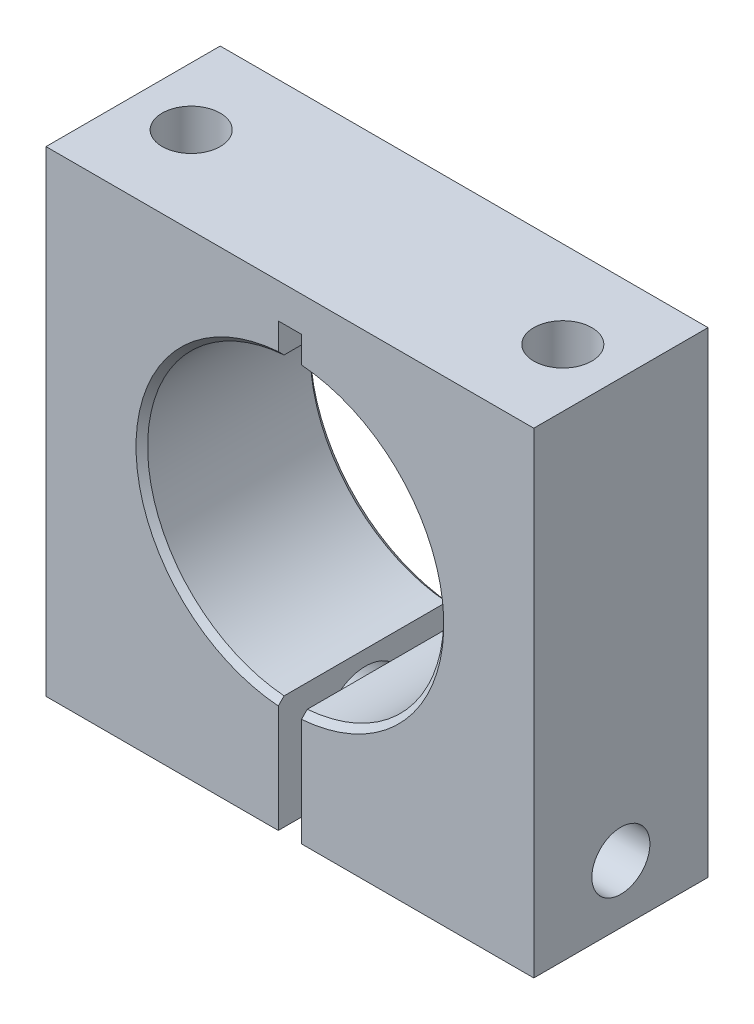
from build123d import *

# Parameters (mm, degrees)
SKETCH_1_W                = 42
SKETCH_1_H                = 41
EXTRUDE_1_DEPTH           = 15
SKETCH_2_R                = 12.75
CUT_EXTRUDE_1_DEPTH       = 15
SKETCH_3_W                = 2
SKETCH_3_H                = 38
CUT_EXTRUDE_2_DEPTH       = 15
HOLE_WIZARD_M6_1_D        = 5
HOLE_WIZARD_M6_1_DEPTH    = 17
HOLE_WIZARD_M6_1_TIP      = 1.502151548
HOLE_WIZARD_7_0_7_1_D     = 7
HOLE_WIZARD_7_0_7_1_DEPTH = 20
HOLE_WIZARD_M6_2_D        = 5
CHAMFER_1_SIZE            = 0.5
CHAMFER_2_SIZE            = 0.5


with BuildPart() as part:
    # 草图1 → 凸台-拉伸1 (new body)
    with BuildSketch(Plane.XY):
        with Locations((21, 20.5)):
            Rectangle(SKETCH_1_W, SKETCH_1_H)
    extrude(amount=EXTRUDE_1_DEPTH)

    # 草图2 → 切除-拉伸1 (cut)
    with BuildSketch(Plane.XY.offset(15)):
        with Locations((21, 22.5)):
            Circle(SKETCH_2_R)
    extrude(amount=-CUT_EXTRUDE_1_DEPTH, mode=Mode.SUBTRACT)

    # 草图3 → 切除-拉伸2 (cut)
    with BuildSketch(Plane.XY.offset(15)):
        with Locations((21, 19)):
            Rectangle(SKETCH_3_W, SKETCH_3_H)
    extrude(amount=-CUT_EXTRUDE_2_DEPTH, mode=Mode.SUBTRACT)

    # M6 螺纹孔1
    with Locations(Plane(origin=(0, 41, 0), x_dir=(1, 0, 0), z_dir=(0, 1, 0))):
        with Locations((5, -7.5), (37, -7.5)):
            Hole(HOLE_WIZARD_M6_1_D / 2, depth=HOLE_WIZARD_M6_1_DEPTH)
            with Locations((0, 0, -(HOLE_WIZARD_M6_1_DEPTH + HOLE_WIZARD_M6_1_TIP / 2))):  # 118° drill point
                Cone(0, HOLE_WIZARD_M6_1_D / 2, HOLE_WIZARD_M6_1_TIP, mode=Mode.SUBTRACT)

    # Ø7.0 (7) 直径孔1
    with Locations(Plane.ZY):
        with Locations((7.5, 5)):
            Hole(HOLE_WIZARD_7_0_7_1_D / 2, depth=HOLE_WIZARD_7_0_7_1_DEPTH)

    # M6 螺纹孔2 (through all)
    with Locations(Plane.ZY.offset(-22)):
        with Locations((7.5, 5)):
            Hole(HOLE_WIZARD_M6_2_D / 2)

    # 倒角1
    chamfer_1_edges = [part.edges().sort_by_distance(p)[0] for p in [
        (33.75, 22.5, 0),
        (33.75, 22.5, 15),
    ]]
    chamfer(chamfer_1_edges, length=CHAMFER_1_SIZE)

    # 倒角2
    chamfer_2_edges = [part.edges().sort_by_distance(p)[0] for p in [
        (8.25, 22.5, 0),
        (8.25, 22.5, 15),
    ]]
    chamfer(chamfer_2_edges, length=CHAMFER_2_SIZE)


solid = part.part
